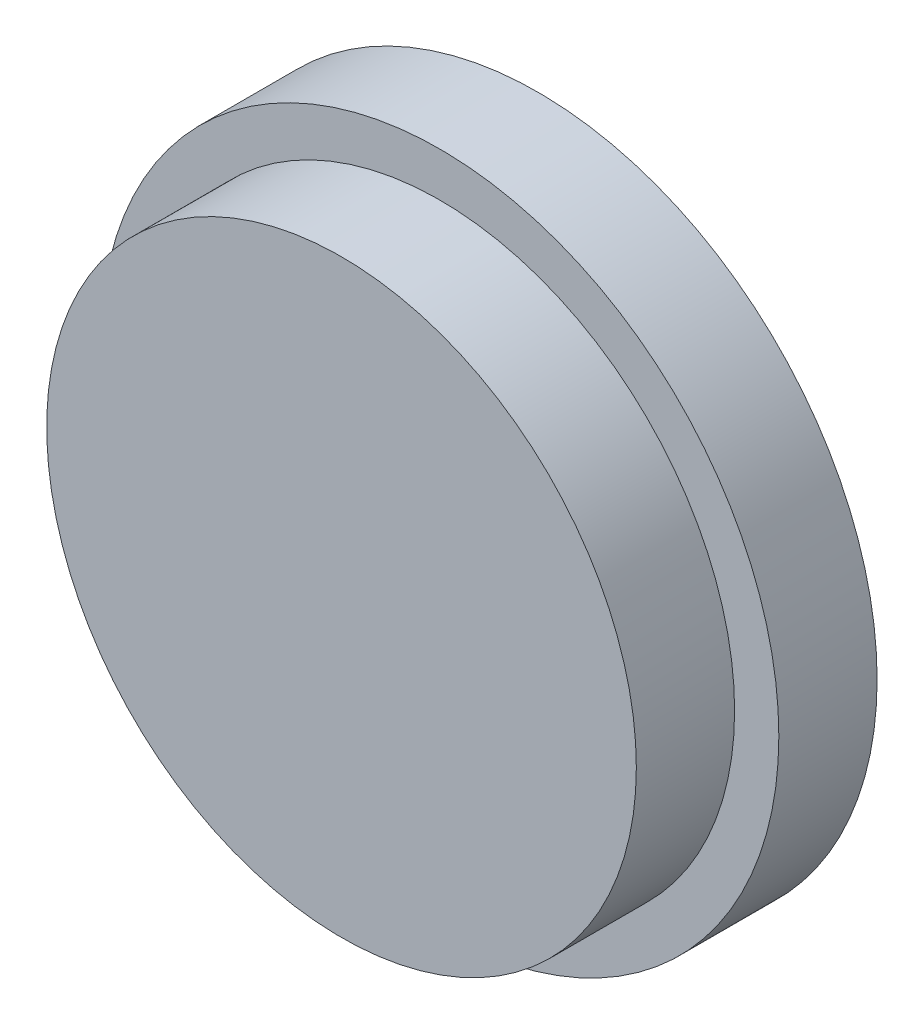
from build123d import *

# Parameters (mm, degrees)
SKETCH_1_3_R        = 3
BOSS_EXTRUDE1_DEPTH = 1
SKETCH_1_3_2_R      = 3.45
BOSS_EXTRUDE2_DEPTH = 1


with BuildPart() as part:
    # Sketch 1_3 → Boss-Extrude1 (new body)
    with BuildSketch(Plane.XY):
        Circle(SKETCH_1_3_R)
    extrude(amount=BOSS_EXTRUDE1_DEPTH)

    # Sketch 1_3 2 → Boss-Extrude2 (add)
    with BuildSketch(Plane.XY):
        Circle(SKETCH_1_3_2_R)
    extrude(amount=-BOSS_EXTRUDE2_DEPTH)


solid = part.part
